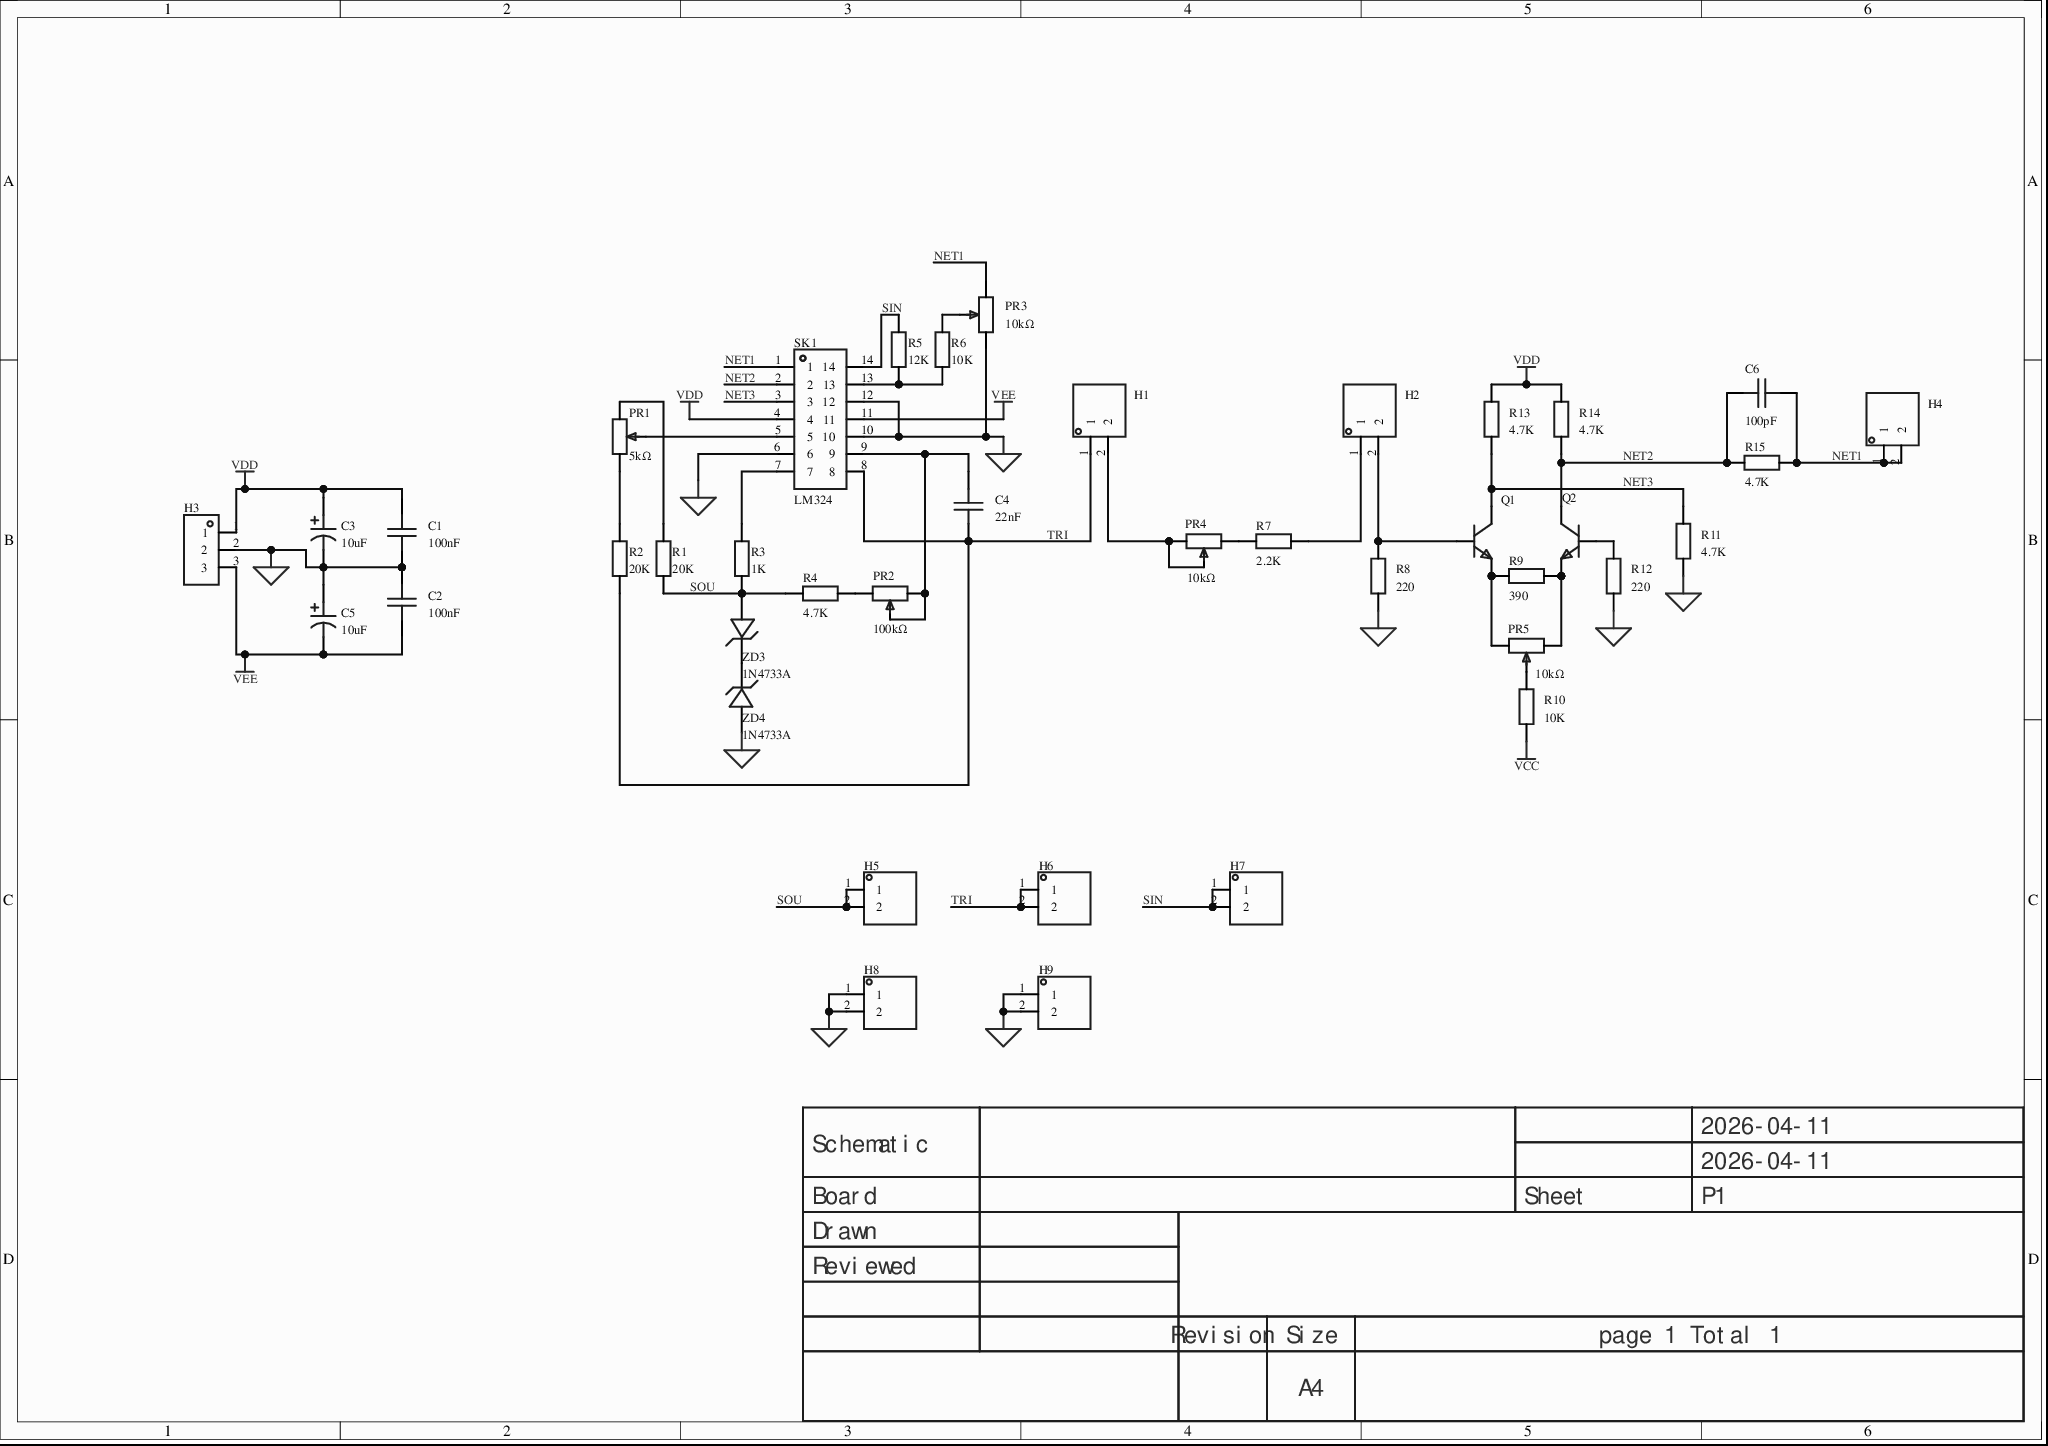
[diagram p0: MISC51604-3.schdoc]
# Altium project MISC51604-2.PrjPcb
1 sheet, 40 parts. Net scope: global (net labels, ports and power ports of the same name join across sheets).
Board file: MISC51604.pcbdoc

## Sheet MISC51604-3.schdoc
size 297 x 209 mm; Version: V1.0; @Project Name: MISC51604; @Update Date: 2026-04-11; @Create Date: 2026-04-11; @Board Name: MISC51604; @Create Time: 14:26:21; @Page Count: 1; @Page No: 1; @Schematic Name: MISC51604; @Update Time: 14:26:21; Size: A4

### Parts
C1  100nF  [L0805]
C2  100nF  [L0805]
C3  10uF  [CAP-TH_BD5.0-P2.00-D0.5-FD-A]
C4  22nF  [C0805]
C5  10uF  [CAP-TH_BD5.0-P2.00-D0.5-FD-A]
C6  100pF  [C0805]
H1  (no value)  [HDR-TH_2P-P2.54-V-M-1]
H2  (no value)  [HDR-TH_2P-P2.54-V-M-1]
H3  (no value)  [CONN-TH_3P-P2.50_HX-XH2.54-3PZZ-B]
H4  (no value)  [HDR-TH_2P-P2.54-V-M-1]
H5  (no value)  [HDR-TH_2P-P2.54-V-M-1]
H6  (no value)  [HDR-TH_2P-P2.54-V-M-1]
H7  (no value)  [HDR-TH_2P-P2.54-V-M-1]
H8  (no value)  [HDR-TH_2P-P2.54-V-M-1]
H9  (no value)  [HDR-TH_2P-P2.54-V-M-1]
PR1  5kΩ  [R_3296]
PR2  100kΩ  [R_3296]
PR3  10kΩ  [R_3296]
PR4  10kΩ  [R_3296]
PR5  10kΩ  [R_3296]
Q1  (no value)  [S8050_TO_92]
Q2  (no value)  [S8050_TO_92]
R1  20K  [R0805]
R2  20K  [R0805]
R3  1K  [R0805]
R4  4.7K  [R0805]
R5  12K  [R0805]
R6  10K  [R0805]
R7  2.2K  [R0805]
R8  220  [R0805]
R9  390  [R0805]
R10  10K  [R0805]
R11  4.7K  [R0805]
R12  220  [R0805]
R13  4.7K  [R0805]
R14  4.7K  [R0805]
R15  4.7K  [R0805]
SK1  LM324  [DIP-14_L17.8-W10.2-P2.54-BL]
ZD3  1N4733A  [DO-41_BD2.8-L4.2-P8.00-D0.7-FD]
ZD4  1N4733A  [DO-41_BD2.8-L4.2-P8.00-D0.7-FD]

### Nets
GND: C1.1 C2.2 C3.2 C5.1 H3.2 H8.1 H8.2 H9.1 H9.2 PR3.3 R8.1 R11.1 R12.1 SK1.6 SK1.10 SK1.12 ZD4.1(A)
VCC: R10.1
VDD: C1.2 C3.1 H3.1 R13.2 R14.2 SK1.4
VEE: C2.1 C5.2 H3.3 SK1.11
NET1: C6.2 H4.1 H4.2 PR3.1 R15.1 SK1.1
NET2: C6.1 Q2.3(C) R14.1 R15.2 SK1.2
NET3: Q1.3(C) R11.2 R13.1 SK1.3
SIN: H7.1 H7.2 R5.2 SK1.14
SOU: H5.1 H5.2 R1.1 R3.1 R4.2 ZD3.1(A)
TRI: C4.1 H1.1 H6.1 H6.2 R2.1 SK1.8
NetC4_2: C4.2 PR2.2 PR2.3 SK1.9
NetH1_2: H1.2 PR4.1 PR4.2
NetH2_1: H2.1 R7.2
NetH2_2: H2.2 Q1.2(B) R8.2
NetPR1_1: PR1.1 R2.2
NetPR1_2: PR1.2 SK1.5
NetPR1_3: PR1.3 R1.2
NetPR2_1: PR2.1 R4.1
NetPR3_2: PR3.2 R6.2
NetPR4_3: PR4.3 R7.1
NetPR5_1: PR5.1 Q1.1(E) R9.1
NetPR5_2: PR5.2 R10.2
NetPR5_3: PR5.3 Q2.1(E) R9.2
NetQ2_2: Q2.2(B) R12.2
NetR3_2: R3.2 SK1.7
NetR5_1: R5.1 R6.1 SK1.13
NetZD3_2: ZD3.2(K) ZD4.2(K)

### Notes on the sheet
- 2026-04-11
- Schematic
- Board
- Sheet
- P1
- Drawn
- Reviewed
- Revision
- Size
- A4
- page 1 Total 1

### Library data of the parts
C1 C2 = CAP_0603: Symbol: Capacitance; 3D Model: ac125912035d415993ca9572d50418b10819f05c4eef4c71ace90d822a990e87; 3D Model Transform: 62.992,31.496,0,0,0,0,0,0,0; ConvertToPcb: yes; ModelName: C0603_L1.6-W0.8-H0.8; Device: CAP_0603; Supplier Footprint: 0603; Value: 100nF; AddInBom: yes; FootprintName: L0805
C3 C5 = ERG50V10M5X11: Capacitance:10uF;Tolerance:±20%;Rated voltage:50V;Ripple current:180mA@100kHz;Equivalent series resistance (ESR):1.3Ω@100kHz;; Manufacturer: JIERR(捷而瑞); 3D Model: 230b3bd6484f4b52b9cf74c8bd6c61990819f05c4eef4c71ace90d822a990e87; 3D Model Transform: 197.2437,197.23953,0,0,0,0,0,0,-196.85; Tolerance: ±20%; Voltage Rating: 50V; Pin Spacing: 2mm; Lifetime: 2000hrs@105℃; AddInBom: yes; Symbol: ERG50V10M5X11; Device: ERG50V10M5X11; LCSC Part Name: 10uF ±20% 50V; Supplier Part: C47344184; Manufacturer Part: ERG50V10M5X11; Supplier Footprint: 插件,D5xL11mm; JLCPCB Part Class: Extended Part; Datasheet: https://item.szlcsc.com/datasheet/ERG50V10M5X11/49556625.html; Supplier: LCSC; Value: 10uF; Ripple Current: 180mA@100kHz; Equivalent Series Resistance(ESR): 1.3Ω@100kHz; Diameter: 5mm; Height - Seated (Max): 11mm; Operating Temperature: -40℃~+105℃; ConvertToPcb: yes; FootprintName: CAP-TH_BD5.0-P2.00-D0.5-FD-A; ModelName: CAP-TH_BD5.0-P2.00-D0.5-FD-A
C4 C6 = CAP_0805: Symbol: Capacitance; 3D Model: 1ba041120af144c991958decab20d2410819f05c4eef4c71ace90d822a990e87; 3D Model Transform: 78.74,51.181,0,0,0,0,0,0.0005,0; ConvertToPcb: yes; ModelName: C0805_L2.0-W1.3-H1.3; Device: CAP_0805; Supplier Footprint: 0805; AddInBom: yes; FootprintName: C0805
  C4: Value: 22nF
  C6: Value: 100pF
H1 H2 H4-H9 = HDR-M_2.54_1x2P: Symbol: 210S-1*2P L=11.6MMGold-plated black; ConvertToPcb: yes; ModelId: 79b2e9f2d70a4d68a1b7098f27c6d4c50819f05c4eef4c71ace90d822a990e87; ModelName: HDR-M-2.54_1x2; ModelTransform: 200,100,0,0,0,0,0,0,-118.11; Device: HDR-M_2.54_1x2P; AddInBom: yes; SupplierPart: C124375; Supplier Footprint: 插件; FootprintName: HDR-TH_2P-P2.54-V-M-1
H3 = HDR-M_2.54_1x3P: 3D Model: bb473b6d38ff42a99216a4fcdbdcc4cb0819f05c4eef4c71ace90d822a990e87; 3D Model Transform: 300.03877,100,0,0,0,0,0,0,-118.11; AddInBom: yes; ModelName: HDR-TH_3P-P2.54-M-LI-1X3P; Symbol: HDR-M_2.54_1x3P; Device: HDR-M_2.54_1x3P; Supplier Part: C2937625; Supplier Footprint: 插件; FootprintName: CONN-TH_3P-P2.50_HX-XH2.54-3PZZ-B; ConvertToPcb: yes
PR1-PR5 = R_3296: ConvertToPcb: yes; ModelId: b182808559bb43bda9e7de64b64134cb0819f05c4eef4c71ace90d822a990e87; ModelName: 3296W; ModelTransform: 373.98,188.96,590.49,180,0,0,0,0,-140; Symbol: R_3296; Device: R_3296; AddInBom: yes; Supplier Footprint: 直插; FootprintName: R_3296
  PR1: Value: 5kΩ
  PR2: Value: 100kΩ
  PR3-PR5: Value: 10kΩ
Q1 Q2 = S8050_TO_NPN: ConvertToPcb: yes; ModelId: aafe8e06f2154e7c93506efd0d6632dd0819f05c4eef4c71ace90d822a990e87; ModelName: TO-92-3_L4.9-W3.7-P1.27-L; ModelTransform: 180.78,141.44,417.3,0,0,0,0,0,-200; Symbol: S8050_TO_NPN; Device: S8050_TO_NPN; AddInBom: yes; Supplier Footprint: TO-92; FootprintName: S8050_TO_92
R1-R15 = Res_0805: Symbol: Resistor; ConvertToPcb: yes; ModelId: 37a81e68749a4138bd2dfa6897b24b850819f05c4eef4c71ace90d822a990e87; ModelName: R0805_L2.0-W1.3-H0.6; ModelTransform: 78.74,51.181,0,0,0,0,0,-0.0005,0; Device: Res_0805; AddInBom: yes; Supplier Footprint: 0805; FootprintName: R0805
  R1 R2: Value: 20K
  R3: Value: 1K
  R4 R11 R13-R15: Value: 4.7K
  R5: Value: 12K
  R6 R10: Value: 10K
  R7: Value: 2.2K
  R8 R12: Value: 220
  R9: Value: 390
SK1 = Z-ICS0S14P-NG00: Adapted package type:DIP;Pitch:2.54mm;Row spacing:7.62mm;Round/square hole:Square hole;Total PIN count:14P;Contact plating:Tin;Operating temperature:-55℃~+105℃;; Manufacturer: Ckmtw(灿科盟); Symbol: ICS-14P; AddInBom: yes; ModelId: cc09d053368342e4bb2f4346b4d2cc000819f05c4eef4c71ace90d822a990e87; ModelName: DIP-14_L17.8-W10.2-H5.1-P2.54; ModelTransform: 699.9986,399.999,0,0,0,0,0,0,-137.795; Adaptation Package Type: DIP; Pitch: 2.54mm; Row Spacing: 7.62mm; Number of Positions: 14P; Device: Z-ICS0S14P-NG00; Manufacturer Part: LM324; LCSC Part Name: 间距2.54mm 方孔 P数:14P; SupplierPart: C132508; Supplier Footprint: DIP-14; JLCPCB Part Class: Extended Part; Datasheet: https://item.szlcsc.com/datasheet/Z-ICS0S14P-NG00/143807.html; Supplier: LCSC; ConvertToPcb: yes; FootprintName: DIP-14_L17.8-W10.2-P2.54-BL; Circular Holes/Square Holes: Square hole; Contact Plating: Tin; Operating Temperature: -55℃~+105℃
ZD3 ZD4 = 1N4733A: Diode configuration:Single;Zener voltage (nominal):5.1V;Zener voltage (range):4.84V~5.36V;Power dissipation (Pd):1W;; Manufacturer: ST(先科); Symbol: 1N4733A_C2536; AddInBom: yes; ModelId: 60a9ba1ea4e145a09c5109b7504cfdbe0819f05c4eef4c71ace90d822a990e87; ModelName: DO-41_D2.8-L4.2-P8.00; ModelTransform: 346.456,102.309,0,180,0,0,0,0,-137.795; Diode Configuration: Single; Zener Voltage(Nom): 5.1V; Reverse Leakage Current (Ir): 10uA@1V; Pd - Power Dissipation: 1W; Impedance(Zzt): 7Ω; Impedance(Zzk): 550Ω; Device: 1N4733A; LCSC Part Name: 停产 1N4733A; SupplierPart: C2536; ManufacturerPart: 1N4733A; Supplier Footprint: DO-41; JLCPCB Part Class: Extended Part; Datasheet: https://item.szlcsc.com/datasheet/1N4733A/2913.html; Supplier: LCSC; ConvertToPcb: yes; FootprintName: DO-41_BD2.8-L4.2-P8.00-D0.7-FD; Zener Voltage(Range): 4.84V~5.36V